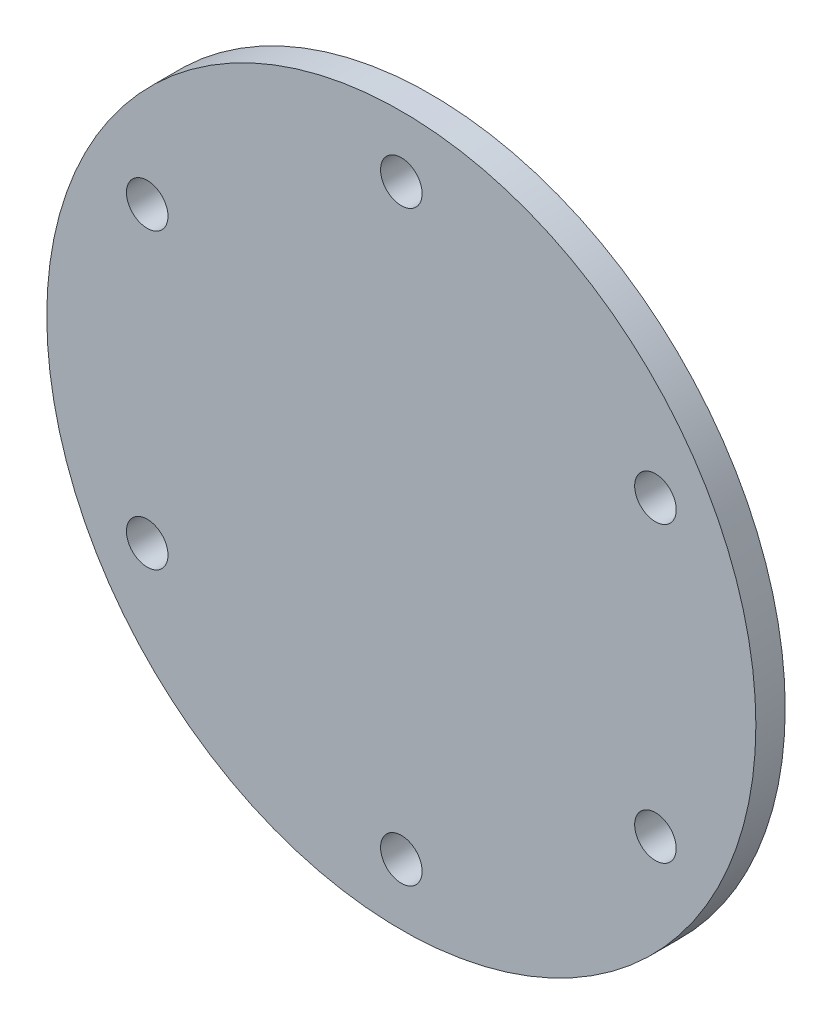
SolidWorks part; units mm, degrees
material "Q235B"
ref_plane "Front Plane" through (0, 0, 0) normal (0, 0, 1) x (1, 0, 0)
ref_plane "Top Plane" through (0, 0, 0) normal (0, 1, 0) x (1, 0, 0)
ref_plane "Right Plane" through (0, 0, 0) normal (1, 0, 0) x (0, 0, -1)
sketch "Sketch1" plane through (0, 0, 0) normal (0, 0, 1) x (1, 0, 0)
  circle A0 centre (0, 0) radius 72.5
  circle A2 centre (0, 60) radius 4.25
  circle A3 centre (51.9615, 30) radius 4.25
  circle A4 centre (51.9615, -30) radius 4.25
  circle A5 centre (0, -60) radius 4.25
  circle A6 centre (-51.9615, -30) radius 4.25
  circle A7 centre (-51.9615, 30) radius 4.25
  point P19 (0, 0)
  dimension "D1" = 6
  dimension "D2" = 145
  dimension "D4" = 8.5
  dimension "D3" = 60
extrude "Boss-Extrude1" add sketch "Sketch1" along normal blind 6
